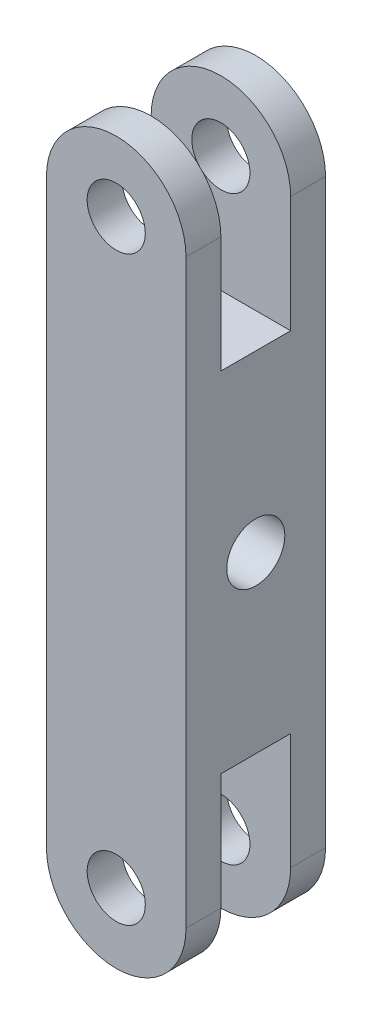
SolidWorks part; units mm, degrees
ref_plane "Front Plane" through (0, 0, 0) normal (0, 0, 1) x (1, 0, 0)
ref_plane "Top Plane" through (0, 0, 0) normal (0, 1, 0) x (1, 0, 0)
ref_plane "Right Plane" through (0, 0, 0) normal (1, 0, 0) x (0, 0, -1)
other "Configuration Table"
sketch "Sketch1" plane through (0, 0, 0) normal (0, 0, 1) x (1, 0, 0)
  line L0 (0, 0) -> (0, 50) construction
  line L1 (-6, 0) -> (-6, 50)
  line L2 (6, 0) -> (6, 50)
  arc A0 (-6, 0) -> (6, 0) centre (0, 0) ccw
  arc A1 (6, 50) -> (-6, 50) centre (0, 50) ccw
  point P3 (0, 25)
  dimension "D1" = 50
  dimension "D2" = 12
extrude "Boss-Extrude1" add sketch "Sketch1" along normal blind 12
sketch "Sketch2" plane through (-6, 0, 0) normal (-1, 0, 0) x (0, 0, 1)
  line L0 (12, 56) -> (0, 56) construction
  line L1 (3, 72) -> (9, 72)
  line L2 (3, 72) -> (3, 40)
  line L3 (3, 40) -> (9, 40)
  line L4 (9, 72) -> (9, 40)
  line L5 (3, 72) -> (9, 40) construction
  line L6 (3, 40) -> (9, 72) construction
  line L7 (0, 25) -> (26.0389, 25) construction
  line L8 (0, 50) -> (0, 0) construction
  line L9 (3, -22) -> (9, -22)
  line L10 (9, -22) -> (9, 10)
  line L11 (3, -22) -> (3, 10)
  line L12 (3, 10) -> (9, 10)
  point P0 (6, 56)
  dimension "D1" = 6
  dimension "D2" = 30
extrude "Cut-Extrude1" cut sketch "Sketch2" against normal through all
sketch "Sketch3" plane through (0, 0, 12) normal (0, 0, 1) x (1, 0, 0)
  circle A0 centre (0, 50) radius 2.5
  circle A1 centre (0, 0) radius 2.5
  dimension "D1" = 5
extrude "Cut-Extrude2" cut sketch "Sketch3" against normal through all
hole_wizard "M6 Tapped Hole1" positions "3DSketch1" profile "Sketch4" tap size "M6" standard "GB" end condition through all
sketch3d "3DSketch1"
  line L0 (6, 0, 0) -> (6, 50, 0) construction
  point P0 (6, 25, 6)
  dimension "D1" = 6
  dimension "D2" = 15
sketch "Sketch4" plane through (6, 25, 6) normal (0, 1, 0) x (0, 0, -1)
  line L0 (0, 0) -> (0, 12)
  line L1 (0, 12) -> (2.5, 12)
  line L2 (2.5, 12) -> (2.5, 0)
  line L5 (2.5, 0) -> (0, 0)
  line L11 (0, -6.35) -> (0, 107.95) construction
  dimension "通孔螺纹孔钻头直径" = 5
  dimension "通孔螺纹孔钻头深度" = 12
cosmetic thread "Hole thread line 1" parameters "D2"=6
